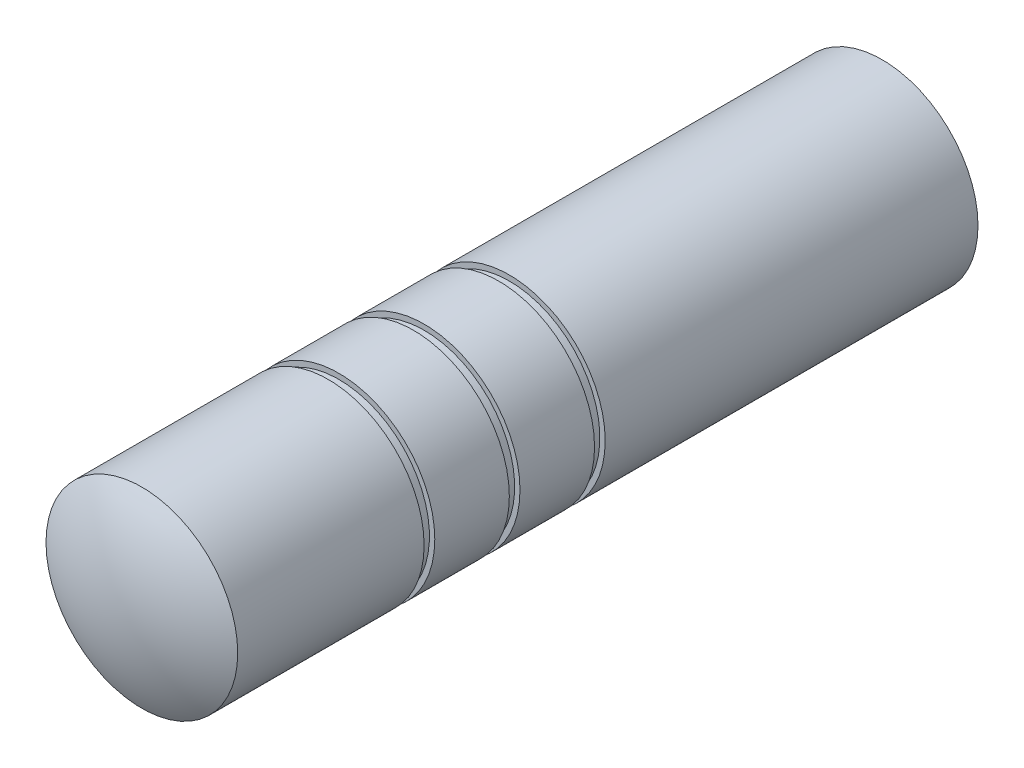
SolidWorks part; units mm, degrees
ref_plane "Front Plane" through (0, 0, 0) normal (0, 0, 1) x (1, 0, 0)
ref_plane "Top Plane" through (0, 0, 0) normal (0, 1, 0) x (1, 0, 0)
ref_plane "Right Plane" through (0, 0, 0) normal (1, 0, 0) x (0, 0, -1)
other "Configuration Table"
sketch "Sketch1" plane through (0, 0, 0) normal (0, 0, 1) x (1, 0, 0)
  circle A0 centre (0, 0) radius 9
  dimension "D1" = 18
extrude "Boss-Extrude1" add sketch "Sketch1" along normal blind 69.5
sketch "Sketch2" plane through (0, 0, 0) normal (0, 0, -1) x (-1, 0, 0)
  circle A0 centre (0, 0) radius 7
  dimension "D1" = 14
extrude "Cut-Extrude1" cut sketch "Sketch2" against normal blind 32
sketch "Sketch3" plane through (0, 0, 0) normal (0, 0, -1) x (-1, 0, 0)
  circle A0 centre (0, 0) radius 9
  circle A1 centre (0, 0) radius 8.5
  dimension "D1" = 18
  dimension "D2" = 17
extrude "Cut-Extrude3" cut sketch "Sketch3" against normal blind 1 from offset 35 offset against normal yes
sketch "Sketch4" plane through (0, 0, 36) normal (0, 0, -1) x (-1, 0, 0)
  circle A0 centre (0, 0) radius 8.5
  circle A1 centre (0, 0) radius 9
  dimension "D1" = 18
  dimension "D2" = 17
extrude "Cut-Extrude4" cut sketch "Sketch4" against normal blind 1 from offset 7 offset against normal yes
sketch "Sketch5" plane through (0, 0, 44) normal (0, 0, -1) x (-1, 0, 0)
  circle A0 centre (0, 0) radius 9
  circle A1 centre (0, 0) radius 8.5
  dimension "D1" = 18
  dimension "D2" = 17
extrude "Cut-Extrude5" cut sketch "Sketch5" against normal blind 1 from offset 7 offset against normal yes
sketch "Sketch6" plane through (0, 0, 0) normal (0, 1, 0) x (1, 0, 0)
  line L0 (0, 0) -> (0, -71.9917) construction
  line L1 (0, -69.5) -> (0, -71.9917)
  line L2 (0, -69.5) -> (-9, -69.5)
  line L3 (-9, -69.5) -> (9, -69.5) construction
  line L4 (7, 0) -> (-7, 0) construction
  arc A0 (-9, -69.5) -> (0, -71.9917) centre (0, -54.4917) ccw
  dimension "D1" = 35
revolve "Revolve1" add sketch "Sketch6" angle 360 about L0
hole_wizard "M5 Tapped Hole1" positions "Sketch7" profile "Sketch8" tap size "M5" standard "GB"
sketch "Sketch7" plane through (0, 0, 32) normal (0, 0, -1) x (-1, 0, 0)
  point P0 (0, 0)
sketch "Sketch8" plane through (0, 0, 32) normal (1, 0, 0) x (0, 1, 0)
  line L0 (0, 0) -> (0, 10)
  line L1 (0, 10) -> (2.1, 8.7382)
  line L2 (2.1, 8.7382) -> (2.1, 0.425)
  line L3 (2.1, 0.425) -> (2.525, 0)
  line L5 (2.525, 0) -> (0, 0)
  line L6 (-2.1, 0.425) -> (-2.525, 0) construction
  line L10 (0, 10) -> (-2.1, 8.7382) construction
  line L11 (0, -6.35) -> (0, 107.95) construction
  dimension "螺纹孔钻头直径" = 4.2
  dimension "螺纹孔钻头深度" = 10
  dimension "近端锥形沉头孔直径" = 5.05
  dimension "近端锥形沉头孔角度" = 90
  dimension "导头角度" = 118
cosmetic thread "Hole Thread1" parameters "D1"=9, "D2"=5
